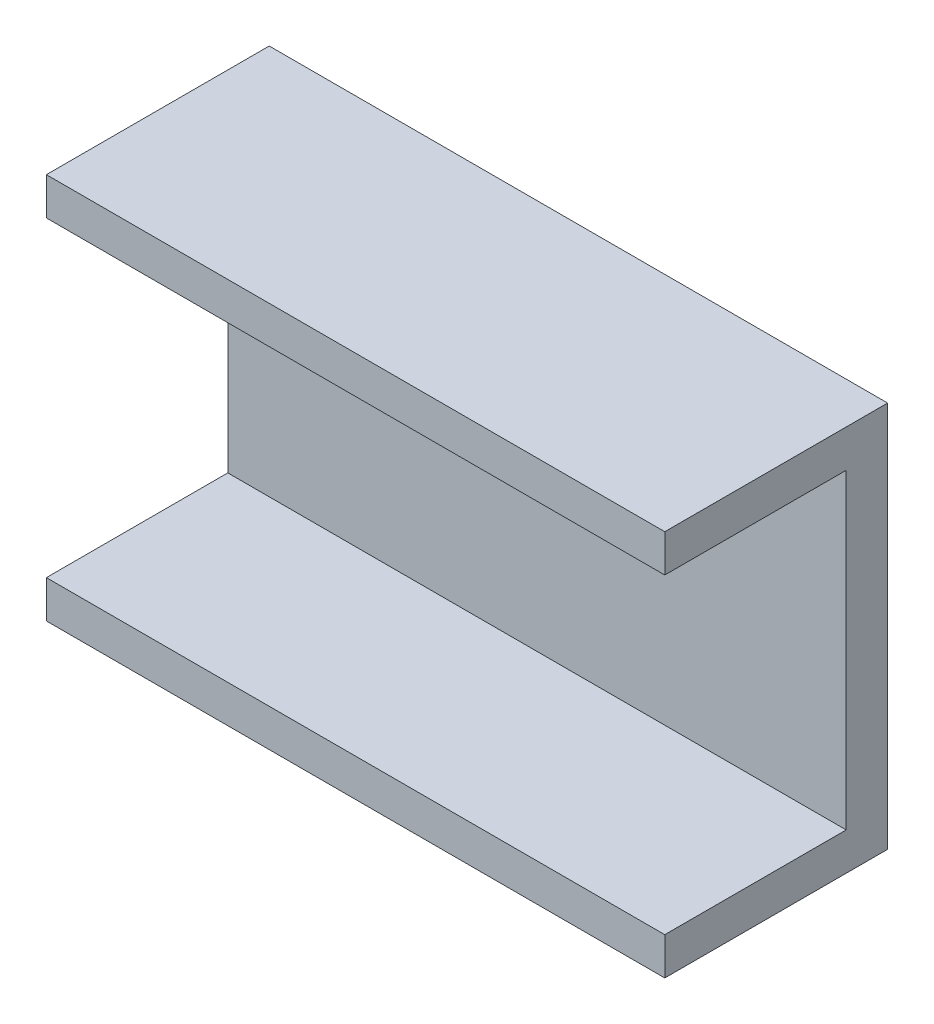
SolidWorks part; units mm, degrees
ref_plane "Front Plane" through (0, 0, 0) normal (0, 0, 1) x (1, 0, 0)
ref_plane "Top Plane" through (0, 0, 0) normal (0, 1, 0) x (1, 0, 0)
ref_plane "Right Plane" through (0, 0, 0) normal (1, 0, 0) x (0, 0, -1)
other "Configuration Table"
sketch "Sketch1" plane through (0, 0, 0) normal (0, 0, 1) x (1, 0, 0)
  line L1 (0, 0) -> (80, 0)
  line L2 (0, 0) -> (0, 50)
  line L3 (0, 50) -> (80, 50)
  line L4 (80, 0) -> (80, 50)
  dimension "D1" = 80
  dimension "D2" = 50
extrude "Boss-Extrude1" add sketch "Sketch1" along normal blind 28.83
sketch "Sketch2" plane through (80, 0, 0) normal (1, 0, 0) x (0, 0, -1)
  line L0 (-28.83, 0) -> (-28.83, 50) construction
  line L1 (-5.3622, 45.1493) -> (-28.83, 45.1493)
  line L2 (-5.3622, 45.1493) -> (-5.3622, 4.8553)
  line L3 (-5.3622, 4.8553) -> (-28.83, 4.8553)
  line L4 (-28.83, 45.1493) -> (-28.83, 4.8553)
extrude "Cut-Extrude1" cut sketch "Sketch2" against normal through all
